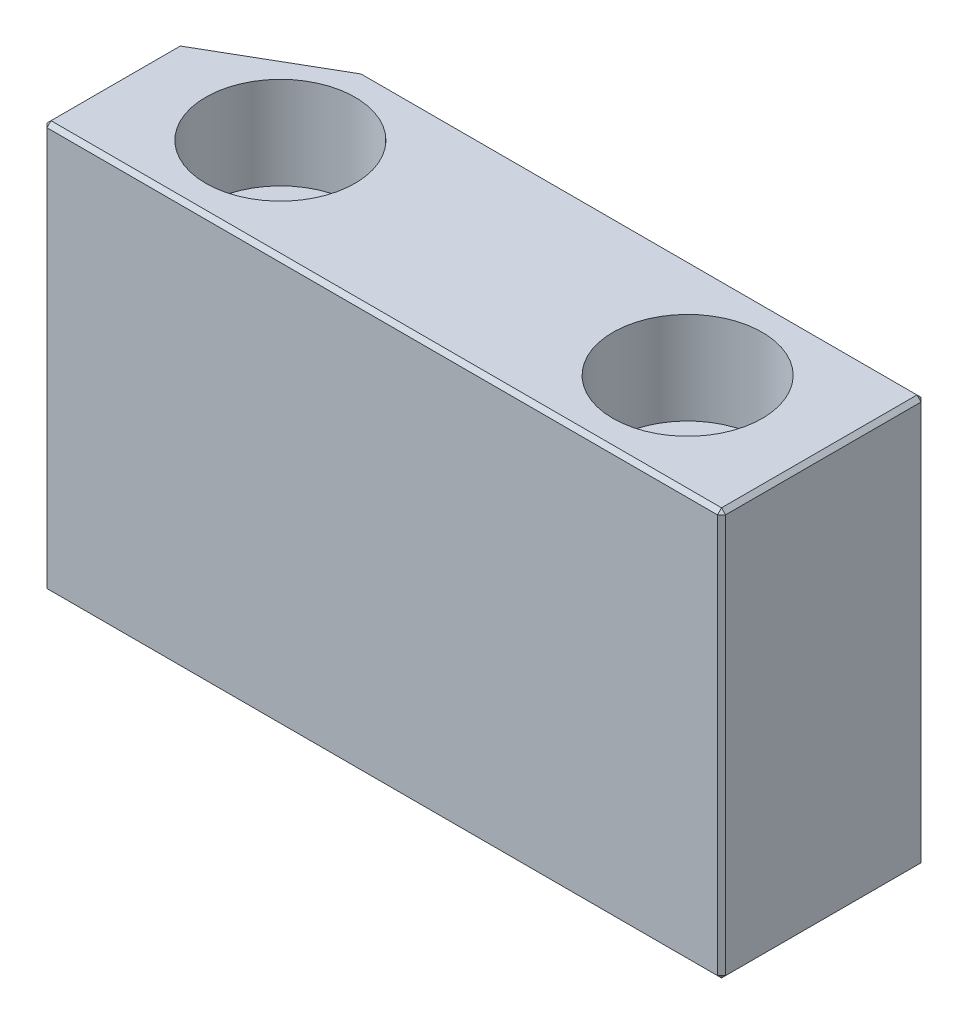
SolidWorks part; units mm, degrees
material "45号钢"
ref_plane "Front" through (0, 0, 0) normal (0, 0, 1) x (1, 0, 0)
ref_plane "Top" through (0, 0, 0) normal (0, 1, 0) x (1, 0, 0)
ref_plane "Right" through (0, 0, 0) normal (1, 0, 0) x (0, 0, -1)
sketch "草图1" plane through (0, 0, 0) normal (0, 0, 1) x (1, 0, 0)
  line L1 (-25, 15) -> (25, 15)
  line L2 (-25, 15) -> (-25, -15)
  line L3 (-25, -15) -> (25, -15)
  line L4 (25, 15) -> (25, -15)
  line L5 (-25, 15) -> (25, -15) construction
  line L6 (-25, -15) -> (25, 15) construction
  point P0 (0, 0)
  dimension "D1" = 50
  dimension "D2" = 30
extrude "凸台-拉伸1" add sketch "草图1" along normal blind 15
hole_wizard "打孔尺寸根据内六角圆柱头螺钉的类型1" positions "草图3" profile "草图2" counterbore size "M6" standard "Gb" end condition through all
sketch "草图3" plane through (0, 15, 0) normal (0, 1, 0) x (1, 0, 0)
  line L0 (25, -7.5) -> (15, -7.5) construction
  line L1 (25, -15) -> (25, 0) construction
  line L3 (0, 0) -> (0, -15) construction
  line L4 (25, -15) -> (-25, -15) construction
  point P0 (-15, -7.5)
  point P2 (15, -7.5)
  dimension "D1" = 30
sketch "草图2" plane through (-15, 15, 7.5) normal (1, 0, 0) x (0, 0, 1)
  line L0 (0, 0) -> (0, 30)
  line L1 (0, 30) -> (3.3, 30)
  line L3 (3.3, 30) -> (3.3, 6.8)
  line L4 (3.3, 6.8) -> (5.5, 6.8)
  line L5 (5.5, 6.8) -> (5.5, 0)
  line L7 (5.5, 0) -> (0, 0)
  line L11 (0, -6.35) -> (0, 107.95) construction
  dimension "通孔孔直径" = 6.6
  dimension "通孔孔深度" = 30
  dimension "柱形沉头孔直径" = 11
  dimension "柱形沉头孔深度" = 6.8
chamfer "倒角1" distance 5 angle 60 1 edges at (-25, 0, 0)
chamfer "倒角2" distance 0.3 angle 45 13 edges at (25, -15, 7.5) (25, 15, 7.5) (25, 0, 0) (0, -15, 15) (4.3301, -15, 0) (-20.6699, -15, 2.5) (-25, -15, 10) (-25, 0, 15) (25, 0, 15) (0, 15, 15) (-25, 15, 10) (-20.6699, 15, 2.5) (4.3301, 15, 0)
